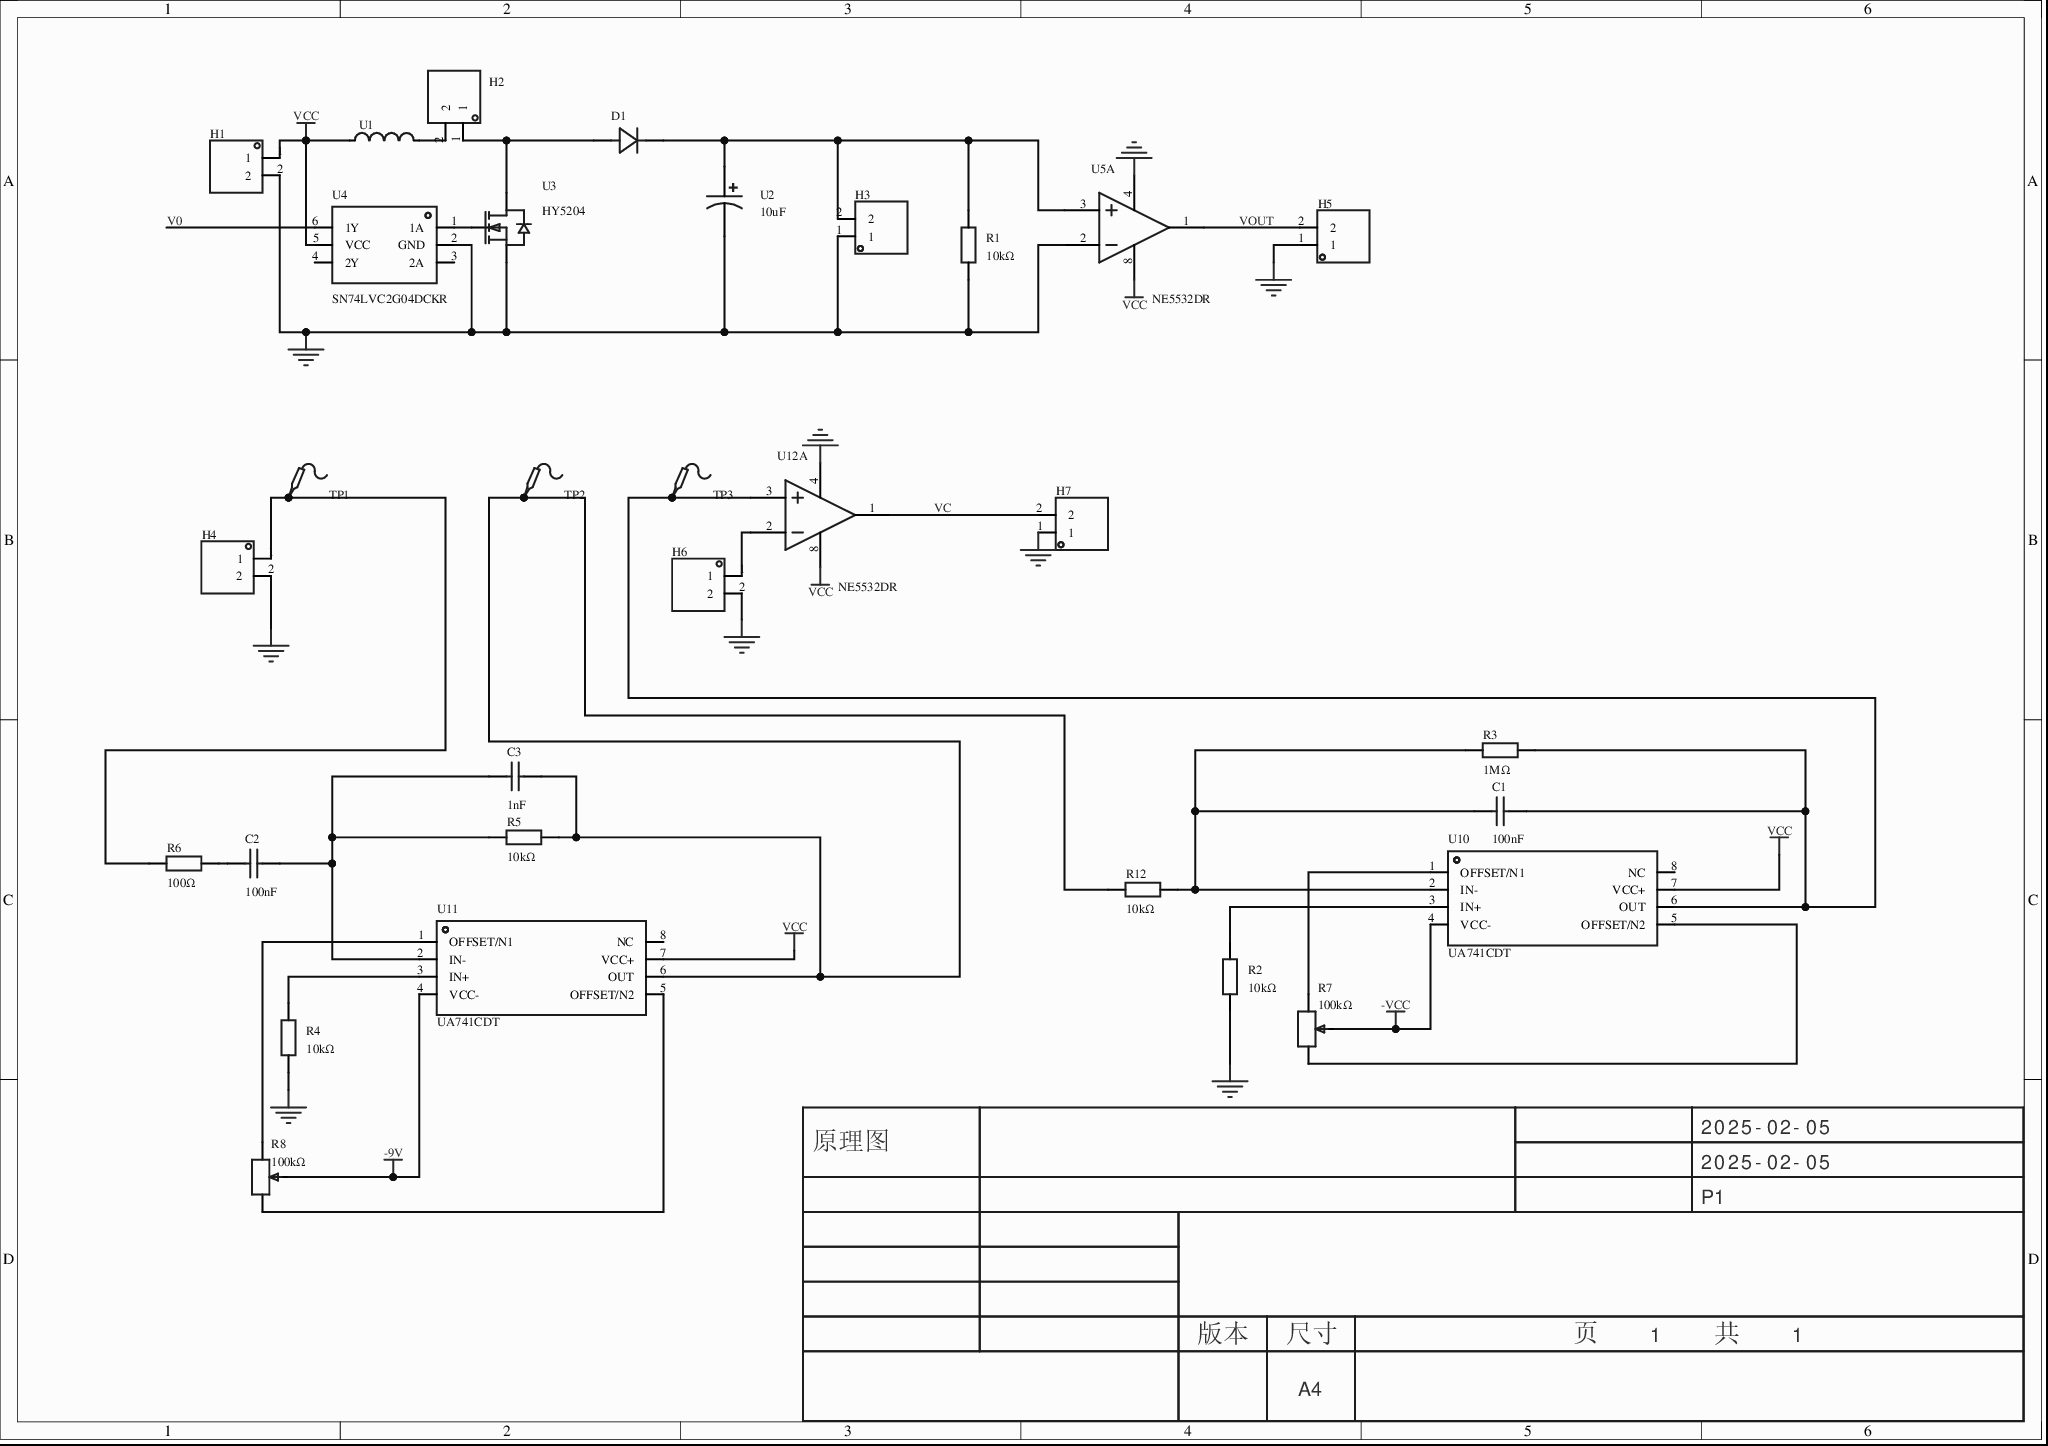
[diagram p0: MISC49892-3.schdoc]
# Altium project MISC49892-2.PrjPcb
1 sheet, 31 parts. Net scope: global (net labels, ports and power ports of the same name join across sheets).
Board file: MISC49892.pcbdoc

## Sheet MISC49892-3.schdoc
size 297 x 209 mm; Version: V1.0; @Project Name: MISC49892; @Page Count: 1; @Update Date: 2025-02-05; @Create Date: 2025-02-05; @Schematic Name: MISC49892; @Page No: 1; @Create Time: 14:09:58; @Update Time: 14:58:38; @Board Name: MISC49892

### Parts
C1  100nF  [C0805]
C2  100nF  [C0805]
C3  1nF  [C0805]
D1  (no value)  [DO_1N4007]
H1  (no value)  [HDR-TH_2P-P2.54-V-M-1]
H2  (no value)  [HDR-TH_2P-P2.54-V-M-1]
H3  (no value)  [HDR-TH_2P-P2.54-V-M-1]
H4  (no value)  [HDR-TH_2P-P2.54-V-M-1]
H5  (no value)  [HDR-TH_2P-P2.54-V-M-1]
H6  (no value)  [HDR-TH_2P-P2.54-V-M-1]
H7  (no value)  [HDR-TH_2P-P2.54-V-M-1]
R1  10kΩ  [Res_1/4W]
R2  10kΩ  [R0805]
R3  1MΩ  [R0805]
R4  10kΩ  [R0805]
R5  10kΩ  [R0805]
R6  100Ω  [R0805]
R7  100kΩ  [RES-ADJ-SMD_VG039NCH]
R8  100kΩ  [RES-ADJ-SMD_VG039NCH]
R12  10kΩ  [R0805]
TP1  (no value)  [Test-Point-0.5mm]
TP2  (no value)  [Test-Point-0.5mm]
TP3  (no value)  [Test-Point-0.5mm]
U1  功率电感(贴片),CKST0502-10uH/M,10uH,±20%,3A,封装5.7mm*5.1mm*2.0mm,岑科,RoHS  [IND-SMD_L5.7-W5.1]  (value not drawn)
U2  10uF  [CAP-TH_BD4.0-P1.50-D0.8-FD]
U3  HY5204  [TO-247-3_L15.8-W5.0-P5.44-L-1]
U4  SN74LVC2G04DCKR  [SOT-363_L2.0-W1.3-P0.65-LS2.1-BR]
U5  NE5532DR  [SOIC-8_L4.9-W3.9-P1.27-LS6.0-BL]  (part A of 2)
U10  UA741CDT  [SOIC-8_L4.9-W3.9-P1.27-LS6.0-BL]
U11  UA741CDT  [SOIC-8_L4.9-W3.9-P1.27-LS6.0-BL]
U12  NE5532DR  [SOIC-8_L4.9-W3.9-P1.27-LS6.0-BL]  (part A of 2)

### Nets
-9V: R8.2 U11.4(VCC-)
-VCC: R7.2 U10.4(VCC-)
GND: H1.2 H3.1 H4.2 H5.1 H6.2 H7.1 R1.1 R2.1 R4.1 U2.2 U3.3(S) U4.2(GND) U5.2(IN1-) U5.4(VCC-/GND) U12.4(VCC-/GND)
VCC: H1.1 U1.1 U4.5(VCC) U5.8(VCC+) U10.7(VCC+) U11.7(VCC+) U12.8(VCC+)
V0: U4.6(1Y)
VC: H7.2 U12.1(OUT1)
VOUT: H5.2 U5.1(OUT1)
NetC1_1: C1.1 R3.1 R12.2 U10.2(IN-)
NetC1_2: C1.2 R3.2 TP3.1 U10.6(OUT) U12.3(IN1+)
NetC2_1: C2.1 R6.2
NetC2_2: C2.2 C3.1 R5.1 U11.2(IN-)
NetC3_2: C3.2 R5.2 R12.1 TP2.1 U11.6(OUT)
NetD1_1: D1.1(K) H3.2 R1.2 U2.1 U5.3(IN1+)
NetD1_2: D1.2(A) H2.1 U3.2(D)
NetH2_2: H2.2 U1.2
NetH4_1: H4.1 R6.1 TP1.1
NetH6_1: H6.1 U12.2(IN1-)
NetR2_2: R2.2 U10.3(IN+)
NetR4_2: R4.2 U11.3(IN+)
NetR7_1: R7.1 U10.5(OFFSET/N2)
NetR7_3: R7.3 U10.1(OFFSET/N1)
NetR8_1: R8.1 U11.1(OFFSET/N1)
NetR8_3: R8.3 U11.5(OFFSET/N2)
NetU3_1: U3.1(G) U4.1(1A)

Not connected (* = marked no-connect by the designer): U4 3(2A)* 4(2Y)*; U10 8(NC); U11 8(NC)

### Notes on the sheet
- 2025-02-05
- 原理图
- P1
- 版本
- 尺寸
- A4
- 页    1    共    1

### Library data of the parts
C1-C3 = CC0805KRX7R9BB104: 容值:100nF;精度:±10%;额定电压:50V;材质(温度系数):X7R;; Manufacturer: YAGEO(国巨); AddInBom: yes; ModelId: 1ba041120af144c991958decab20d241; ModelName: C0805_L2.0-W1.3-H1.3; ModelTransform: 78.74,51.181,0,0,0,0,0,0.0005,0; Tolerance: ±10%; Voltage Rated: 50V; Temperature Coefficient: X7R; Symbol: CC0805KRX7R9BB104; Device: CC0805KRX7R9BB104; LCSC Part Name: 100nF ±10% 50V; ManufacturerPart: CC0805KRX7R9BB104; Supplier Footprint: 0805; JLCPCB Part Class: 基础库; Datasheet: https://atta.szlcsc.com/upload/public/pdf/source/20180224/C181747_15194369449651363981.pdf; Supplier: LCSC; ConvertToPcb: yes; FootprintName: C0805
  C1 C2: SupplierPart: C49678; Value: 100nF
  C3: Value: 1nF
D1 = D_1N4007A: AddInBom: yes; ModelId: 6de1e9b71a0d4751b4e9df530304c1a3; ModelName: DO-41_D2.4-L4.7-P8.70; ModelTransform: 373.9,94.4,232.29,0,0,0,0,0,-140; Symbol: D_1N4007; Device: D_1N4007A; Supplier Footprint: DO-41; ConvertToPcb: yes; FootprintName: DO_1N4007
H1-H7 = HDR-M_2.54_1x2P: Symbol: 210S-1*2P L=11.6MMGold-plated black; ConvertToPcb: yes; ModelId: 79b2e9f2d70a4d68a1b7098f27c6d4c5; ModelName: HDR-M-2.54_1x2; ModelTransform: 200,100,0,0,0,0,0,0,-118.11; Device: HDR-M_2.54_1x2P; AddInBom: yes; SupplierPart: C124375; Supplier Footprint: 插件; FootprintName: HDR-TH_2P-P2.54-V-M-1
R1 = Res_AXIAL-1/4W: AddInBom: yes; SymbolName: 电阻; ModelId: 463263665006444ab7a47bd11b0cf956; ModelName: RES-TH_BD2.4-L6.3-P10.30-D0.6; ModelTransform: 427.165,94.32816,0,0,0,0,0,0,-196.85; Device: Res_AXIAL-1/4W; Supplier Footprint: 轴向引线; ConvertToPcb: yes; FootprintName: Res_1/4W; Value: 10kΩ
R2-R6 R12 = 0805W8F1002T5E_C17414: 电阻类型:厚膜电阻;阻值:10kΩ;精度:±1%;功率:125mW;最大工作电压:150V;温度系数:±100ppm/℃;; Manufacturer: UNI-ROYAL(厚声); AddInBom: yes; ModelId: 37a81e68749a4138bd2dfa6897b24b85; ModelName: R0805_L2.0-W1.3-H0.6; ModelTransform: 78.74,51.181,0,0,0,0,0,-0.0005,0; Tolerance: ±1%; Power(Watts): 125mW; Overload Voltage (Max): 150V; Symbol: 0805W8F1002T5E; Device: 0805W8F1002T5E_C17414; Supplier: LCSC; Manufacturer Part: 0805W8F1002T5E; JLCPCB Part Class: 基础库; LCSC Part Name: 10kΩ ±1% 125mW 厚膜电阻; Supplier Footprint: 0805; Datasheet: https://atta.szlcsc.com/upload/public/pdf/source/20200306/C422600_1E6D84923E4A46A82E41ADD87F860B5C.pdf; ConvertToPcb: yes; FootprintName: R0805; Type: 厚膜电阻; Temperature Coefficient: ±100ppm/℃; Operating Temperature Range: -55℃~+155℃
  R2 R4 R5 R12: Supplier Part: C17414; Value: 10kΩ
  R3: Value: 1MΩ
  R6: Value: 100Ω
R7 R8 = VG039NCHXTB201: 阻值:200Ω;精度:±25%;; Manufacturer: HDK(北陆电气); AddInBom: yes; ModelId: ba438d2707b74a9ab8400a10f68363a0; ModelName: RES-ADJ-SMD_3P-L3.8-W3.0-H1.2-P1.90; ModelTransform: 120.0785,161.61385,0,90,0,0,-3.74,-0.118,0; Tolerance: ±25%; Value: 100kΩ; Device: VG039NCHXTB201; Symbol: VG039NCHXTB201; LCSC Part Name: 200Ω ±25%; ManufacturerPart: VG039NCHXTB201; Supplier Footprint: SMD; JLCPCB Part Class: 扩展库; Datasheet: https://atta.szlcsc.com/upload/public/pdf/source/20171123/C145162_15114111014461137838.pdf; Supplier: LCSC; ConvertToPcb: yes; FootprintName: RES-ADJ-SMD_VG039NCH
TP1-TP3 = Test-Point: Test Point 测试点; AddInBom: yes; Device: Test-Point; ConvertToPcb: yes; SymbolName: Test-Point; FootprintName: Test-Point-0.5mm
U1 = 功率电感(贴片),CKST0502-10uH/M,10uH,±20%,3A,封装5.7mm*5.1mm*2.0mm,岑科,RoHS: AddInBom: yes; ModelId: ffd856615f974dd9b1ff3f65e3b3100d; ModelTransform: 224.409,200.787,0,0,0,0,0,-0.591,0; Symbol: 功率电感(贴片),CKST0502-10UH/M,10UH,±20%,3A,封装5.7MM*5.1MM*2.0MM,岑科,ROHS; Device: 功率电感(贴片),CKST0502-10uH/M,10uH,±20%,3A,封装5.7mm*5.1mm*2.0mm,岑科,RoHS; LCSC Part Name: 功率电感(贴片),CKST0502-10uH/M,10uH,±20%,3A,封装5.7mm*5.1mm*2.0mm,岑科,RoHS; SupplierPart: C9900015114; ManufacturerPart: 功率电感(贴片),CKST0502-10uH/M,10uH,±20%,3A,封装5.7mm*5.1mm*2.0mm,岑科,RoHS; Supplier Footprint: 功率电感(贴片),CKST0502-10uH/M,10uH,±20%,3A,封装5.7mm*5.1mm*2.0mm,岑科,RoHS; JLCPCB Part Class: 扩展库; Supplier: LCSC; ConvertToPcb: yes; FootprintName: IND-SMD_L5.7-W5.1; ModelName: IND-SMD_L5.7-W5.1
U2 = 10MS510MEFC4X5: 容值:10uF;精度:±20%;额定电压:10V;纹波电流:16mA@120Hz;; Manufacturer: rubycon(红宝石); AddInBom: yes; ModelId: 8017ea3dd4884afab5fc61dd7898abc1; ModelName: CAP-TH_D4.0-H7.0-P1.5; ModelTransform: 158.2674,157.45008,0,0,0,0,0,0,-137.795; Tolerance: ±20%; Rated Voltage: 10V; φD: 4mm; L: 5mm; Lifetime @ Temp: 1000hrs@85℃; Symbol: 10MS510MEFC4X5; Device: 10MS510MEFC4X5; LCSC Part Name: 10uF ±20% 10V; SupplierPart: C1579578; ManufacturerPart: 10MS510MEFC4X5; Supplier Footprint: 插件,D4xL5mm; JLCPCB Part Class: 扩展库; Datasheet: https://atta.szlcsc.com/upload/public/pdf/source/20210510/C1579578_ABB61F9CFFB4E7371AD0DBD373B61F20.pdf; Supplier: LCSC; ConvertToPcb: yes; FootprintName: CAP-TH_BD4.0-P1.50-D0.8-FD; Value: 10uF; Ripple Current: 16mA@120Hz; Lead Spacing: 1.5mm; Operating Temperature: -40℃~+85℃
U3 = HY5204: AddInBom: yes; ModelId: 27b35664da8045b09b6c38d0310660f0; ModelTransform: 614.17235,196.88937,0,0,0,0,0,7.874,-196.85; Symbol: HY5204; Device: HY5204; LCSC Part Name: HY5204; SupplierPart: C9900006698; ManufacturerPart: HY5204; Supplier Footprint: MOSFET-N; JLCPCB Part Class: 扩展库; Supplier: LCSC; ConvertToPcb: yes; FootprintName: TO-247-3_L15.8-W5.0-P5.44-L-1; ModelName: TO-247-3_L15.8-W5.0-P5.44-L-1
U4 = SN74LVC2G04DCKR: 输入类型:-;电源电压:1.65V~5.5V;供电电流(最大值):10uA;电路数:2;最大传播延迟(tpd):3.2ns@5V,50pF;; Manufacturer: TI(德州仪器); AddInBom: yes; ModelId: ea15c7b026c54341854a7f0d9614aed9; ModelName: SOT-363-6P_L2.0-W1.3-H1.1-LS2.0-P0.65; ModelTransform: 83.17133,78.74,0,180,0,0,0,0,0; Supply Current (Max): 10uA; Number of Circuits: 2; Sink Current: 32mA; High level range (VIH): 1.7V~2V; Low level range (VIL): 700mV~800mV; Symbol: SN74LVC2G04DCKR; Device: SN74LVC2G04DCKR; LCSC Part Name: 双路反相器; SupplierPart: C105251; ManufacturerPart: SN74LVC2G04DCKR; Supplier Footprint: SOT-363-6; JLCPCB Part Class: 扩展库; Datasheet: https://www.ti.com/cn/lit/gpn/sn74lvc2g04; Supplier: LCSC; ConvertToPcb: yes; FootprintName: SOT-363_L2.0-W1.3-P0.65-LS2.1-BR; Input Type: -; Supply Voltage(Single): 1.65V~5.5V; Number of Inputs: 2; Source Current: 32mA; Max Propagation Delay: 3.2ns@5V,50pF; Series: 74LVC系列; Operating Temperature: -40℃~+125℃
U5 U12 = NE5532DR: 放大器数:双路;增益带宽积(GBP):10MHz;输入偏置电流(Ib):200nA;压摆率(SR):9V/us;带宽(-3db):-;; Manufacturer: TI(德州仪器); Relevance: []; AddInBom: yes; ModelId: e81d2f7d937b4a6ab1dca543ff5d56a4; ModelName: SOIC-8_L4.9-W3.9-H1.7-LS6.0-P1.27; ModelTransform: 189.751,236.22,0,0,0,0,0.0005,0.0005,0; Number of Circuits: 双路; Gain Bandwidth Product(GBP): 10MHz; Current - Input Bias(Ib): 200nA; Slew Rate(SR): 9V/us; Output Current: 38mA; Supply Current: 8mA; Symbol: NE5532DR; Device: NE5532DR; LCSC Part Name: NE5532DR; SupplierPart: C7426; ManufacturerPart: NE5532DR; Supplier Footprint: SOIC-8; Datasheet: http://www.ti.com/cn/lit/gpn/ne5532; Supplier: LCSC; ConvertToPcb: yes; FootprintName: SOIC-8_L4.9-W3.9-P1.27-LS6.0-BL; -3db Bandwidth: -; Operating Temperature: 0℃~+70℃
U10 U11 = UA741CDT: 放大器数:单路;增益带宽积(GBP):1MHz;输入偏置电流(Ib):10nA;压摆率(SR):0.5V/us;带宽(-3db):-;; Manufacturer: ST(意法半导体); AddInBom: yes; ModelId: e81d2f7d937b4a6ab1dca543ff5d56a4; ModelName: SOIC-8_L4.9-W3.9-H1.7-LS6.0-P1.27; ModelTransform: 189.751,236.22,0,0,0,0,0.0005,0.0005,0; Number of Circuits: 单路; Gain Bandwidth Product(GBP): 1MHz; Current - Input Bias(Ib): 10nA; Output Current: 25mA; Supply Current: 3.3mA; Symbol: UA741CDT; Device: UA741CDT; LCSC Part Name: UA741CDT; SupplierPart: C7111; ManufacturerPart: UA741CDT; Supplier Footprint: SOIC-8; JLCPCB Part Class: 扩展库; Datasheet: https://atta.szlcsc.com/upload/public/pdf/source/20181030/C283333_E7CFD90DFDEB0B09152BEF9966FA2369.pdf; Supplier: LCSC; ConvertToPcb: yes; FootprintName: SOIC-8_L4.9-W3.9-P1.27-LS6.0-BL; Slew Rate(SR): 0.5V/us; -3db Bandwidth: -; Operating Temperature: 0℃~+70℃